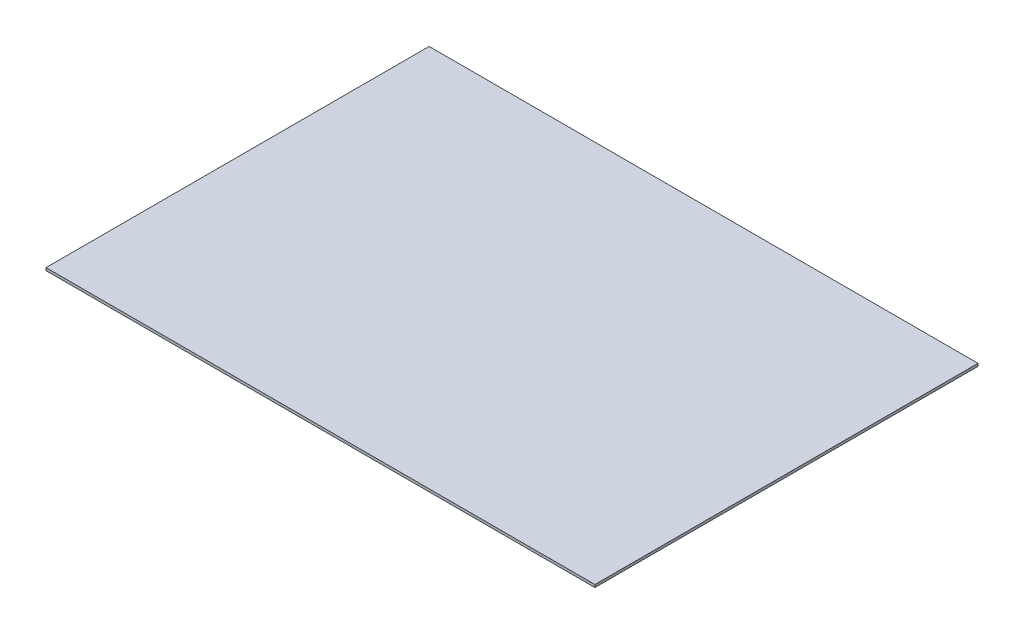
SolidWorks part; units mm, degrees
ref_plane "前视基准面" through (0, 0, 0) normal (0, 0, 1) x (1, 0, 0)
ref_plane "上视基准面" through (0, 0, 0) normal (0, 1, 0) x (1, 0, 0)
ref_plane "右视基准面" through (0, 0, 0) normal (1, 0, 0) x (0, 0, -1)
sketch "草图1" plane through (0, 0, 0) normal (0, 1, 0) x (1, 0, 0)
  line L1 (-207.75, -145) -> (207.75, -145)
  line L2 (-207.75, -145) -> (-207.75, 145)
  line L3 (-207.75, 145) -> (207.75, 145)
  line L4 (207.75, -145) -> (207.75, 145)
  line L5 (-207.75, -145) -> (207.75, 145) construction
  line L6 (-207.75, 145) -> (207.75, -145) construction
  point P0 (0, 0)
  dimension "D1" = 415.5
  dimension "D2" = 290
extrude "凸台-拉伸1" add sketch "草图1" along normal blind 2
